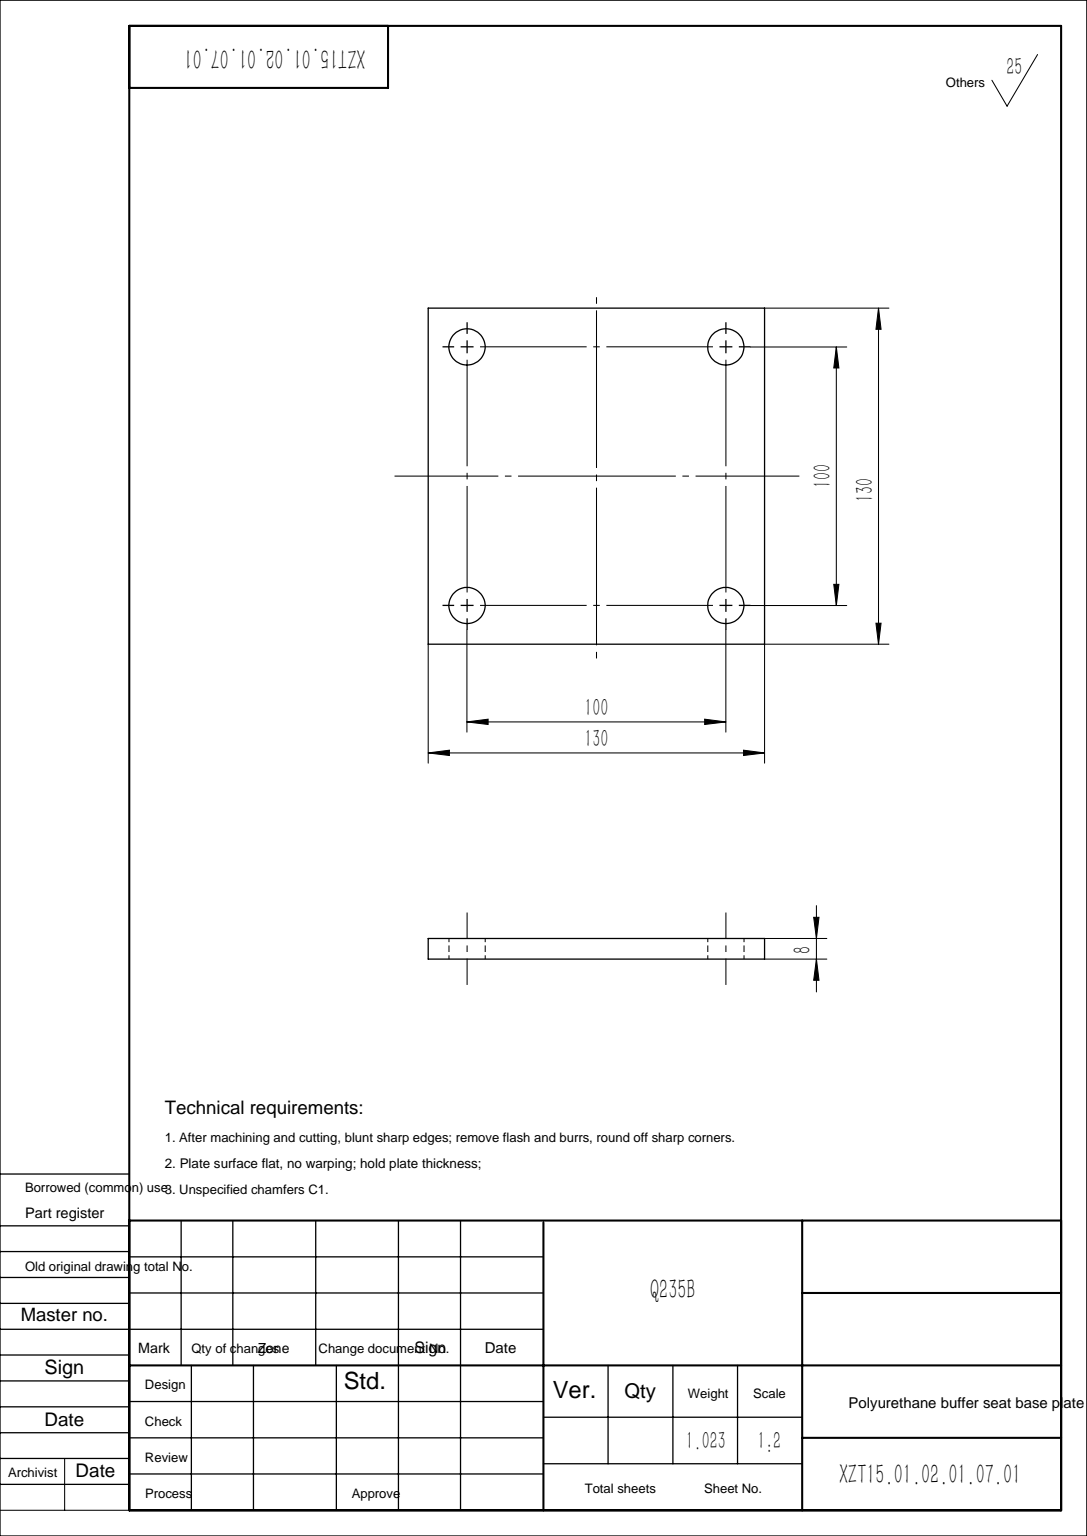
from build123d import *

# Parameters (mm, degrees)
SKETCH1_W                  = 130
SKETCH1_H                  = 130
BOSS_EXTRUDE1_DEPTH        = 8
F_14_0_14_DIAMETER_HOLE1_D = 14


with BuildPart() as part:
    # Sketch1 → Boss-Extrude1 (new body)
    with BuildSketch(Plane(origin=(0, 0, 0), x_dir=(1, 0, 0), z_dir=(0, 1, 0))):
        Rectangle(SKETCH1_W, SKETCH1_H)
    extrude(amount=BOSS_EXTRUDE1_DEPTH)

    # Ø14.0 (14) Diameter Hole1 (through all)
    with Locations(Plane(origin=(0, 8, 0), x_dir=(1, 0, 0), z_dir=(0, 1, 0))):
        with Locations((-50, -50), (50, -50), (50, 50), (-50, 50)):
            Hole(F_14_0_14_DIAMETER_HOLE1_D / 2)


solid = part.part
